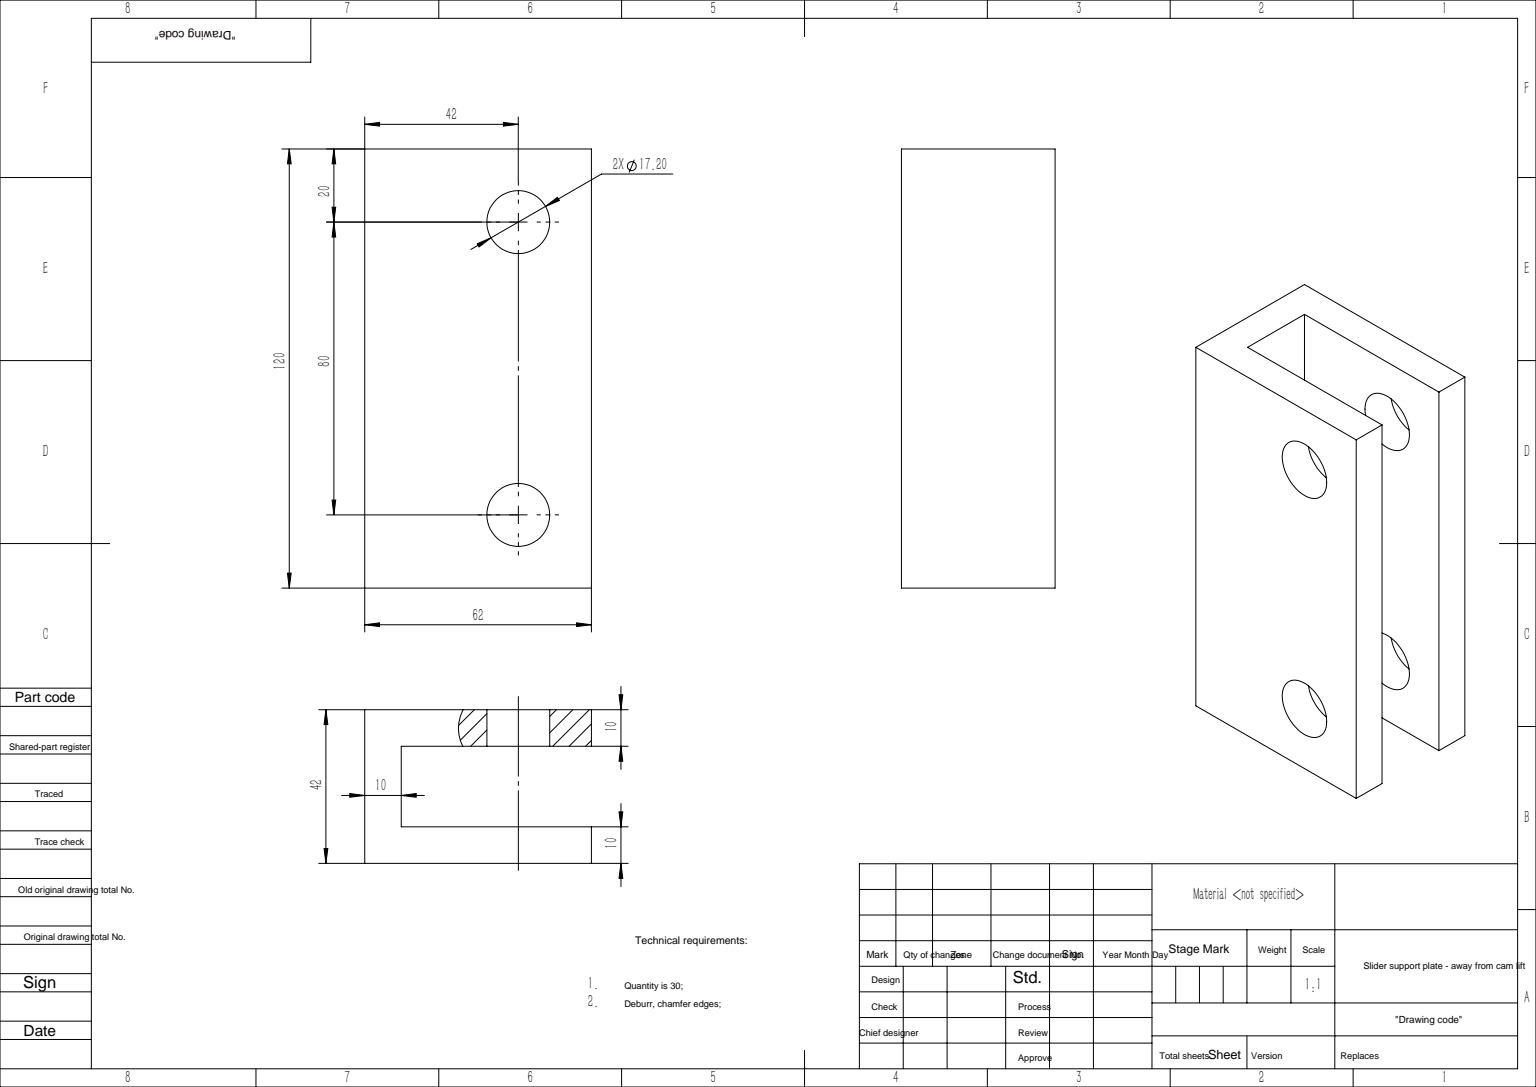
from build123d import *

# Parameters (mm, degrees)
EXTRUDE_1_DEPTH     = 120
SKETCH_2_R          = 8.6
CUT_EXTRUDE_1_DEPTH = 142.449637681


with BuildPart() as part:
    # 草图1 → 凸台-拉伸1 (new body)
    with BuildSketch(Plane(origin=(0, 0, 0), x_dir=(1, 0, 0), z_dir=(0, 1, 0))):
        Polygon((62, 11), (10, 11), (10, -11), (62, -11), (62, -21), (0, -21), (0, 21), (62, 21), align=None)
    extrude(amount=EXTRUDE_1_DEPTH)

    # 草图2 → 切除-拉伸1 (cut, through all)
    with BuildSketch(Plane.XY.offset(21)):
        with Locations((42, 100)):
            Circle(SKETCH_2_R)
        with Locations((42, 20)):
            Circle(SKETCH_2_R)
    extrude(amount=-CUT_EXTRUDE_1_DEPTH, mode=Mode.SUBTRACT)


solid = part.part
